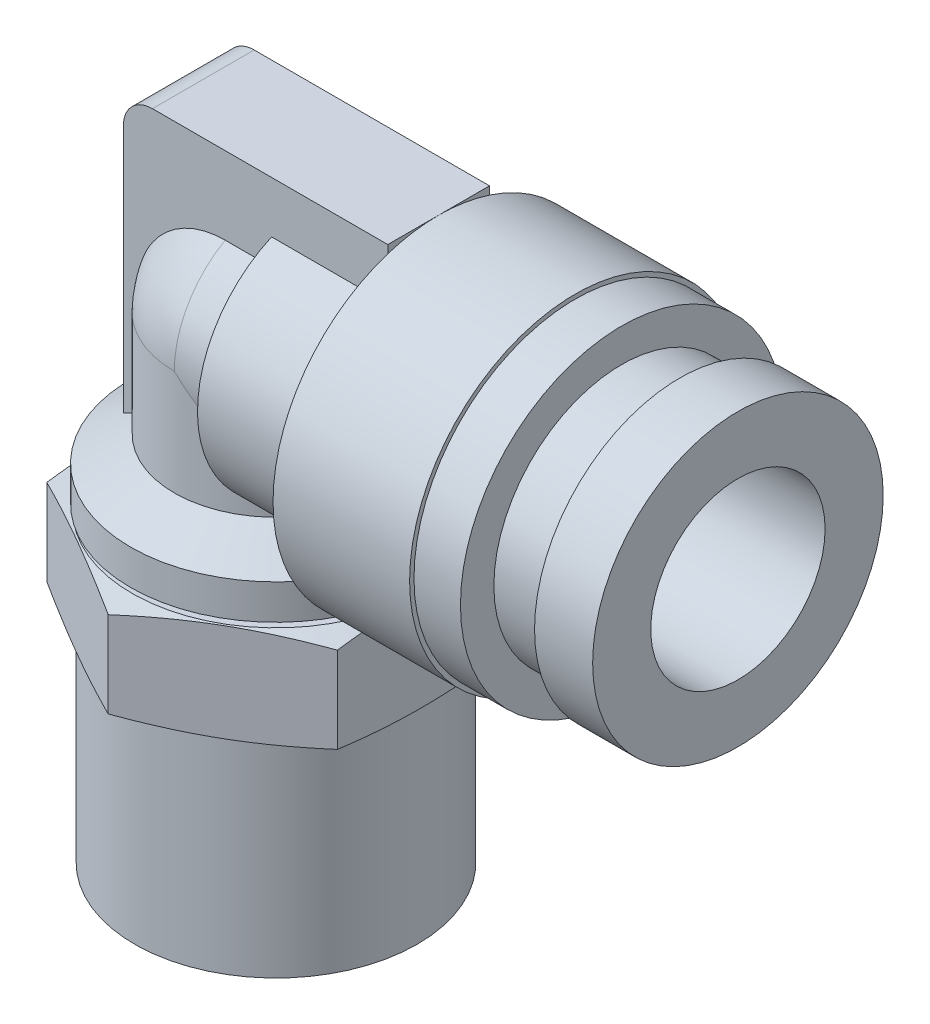
from build123d import *

# Parameters (mm, degrees)
BOSS_EXTRUDE1_DEPTH      = 1.75
BOSS_EXTRUDE1_DEPTH_BACK = 1.75
SKETCH3_R                = 23.447488612
CUT_EXTRUDE1_DEPTH       = 3.4
HOLE1_D                  = 6
HOLE1_DEPTH              = 13.6


with BuildPart() as part:
    # Sketch1 → Revolve1 (revolve)
    with BuildSketch(Plane.XY, mode=Mode.PRIVATE) as revolve1_sk:
        Polygon((0, -3.1), (-4.864, -3.1), (-4.864, 4), (-4.95, 4), (-8, 4.817245037), (-8, 6.582754963), (-4.95, 7.4), (-3.3, 7.4), (-3.3, 7.6), (-5, 7.6), (-5, 8.803974596), (-3.5, 9.67), (-3.5, 13.3), (0, 13.3), align=None)
    revolve(revolve1_sk.sketch.rotate(Axis((0, 13.3, 0), (0, -1, 0)), 180), axis=Axis((0, 13.3, 0), (0, -1, 0)))

    # Sketch2 → Boss-Extrude1 (add, two sides: drawn at the far end of the back side and taken through both)
    with BuildSketch(Plane.XY.offset(-BOSS_EXTRUDE1_DEPTH_BACK)):
        with BuildLine():
            Line((-3.5, 7.6), (5.6, 7.6))
            Line((5.6, 7.6), (5.6, 19))
            Line((5.6, 19), (-2.5, 19))
            ThreePointArc((-2.5, 19), (-3.207106781, 18.707106781), (-3.5, 18))
            Line((-3.5, 18), (-3.5, 7.6))
        make_face()
    extrude(amount=BOSS_EXTRUDE1_DEPTH + BOSS_EXTRUDE1_DEPTH_BACK)

    # Sketch3 → Cut-Extrude1 (cut)
    with BuildSketch(Plane(origin=(0, 7.4, 0), x_dir=(1, 0, 0), z_dir=(0, 1, 0))):
        Circle(SKETCH3_R)
        Polygon((-5, 2.886751346), (-5, -2.886751346), (0, -5.773502692), (5, -2.886751346), (5, 2.886751346), (0, 5.773502692), align=None, mode=Mode.SUBTRACT)
    extrude(amount=-CUT_EXTRUDE1_DEPTH, mode=Mode.SUBTRACT)

    # Sketch4 → Revolve2 (revolve)
    with BuildSketch(Plane.XY, mode=Mode.PRIVATE) as revolve2_sk:
        with BuildLine():
            Line((0, 16.8), (1.138119785, 16.8))
            Line((1.138119785, 16.8), (1.6, 17.6))
            Line((1.6, 17.6), (4.791709623, 17.6))
            Line((4.791709623, 17.6), (5.6, 19))
            Line((5.6, 19), (10.3, 19))
            Line((10.3, 19), (10.3, 18.85))
            Line((10.3, 18.85), (11.9, 18.85))
            Line((11.9, 18.85), (11.9, 17.7))
            Line((11.9, 17.7), (13.9, 17.7))
            Line((13.9, 17.7), (13.9, 18.3))
            Line((13.9, 18.3), (15.9, 18.3))
            Line((15.9, 18.3), (15.9, 13.3))
            Line((15.9, 13.3), (-3.5, 13.3))
            ThreePointArc((-3.5, 13.3), (-2.474873734, 15.774873734), (0, 16.8))
        make_face()
    revolve(revolve2_sk.sketch.rotate(Axis((15.9, 13.3, 0), (-1, 0, 0)), 270), axis=Axis((15.9, 13.3, 0), (-1, 0, 0)))

    # Hole1
    with Locations(Plane(origin=(15.9, 0, 0), x_dir=(0, 0, -1), z_dir=(1, 0, 0))):
        with Locations((0, 13.3)):
            Hole(HOLE1_D / 2, depth=HOLE1_DEPTH)


solid = part.part
